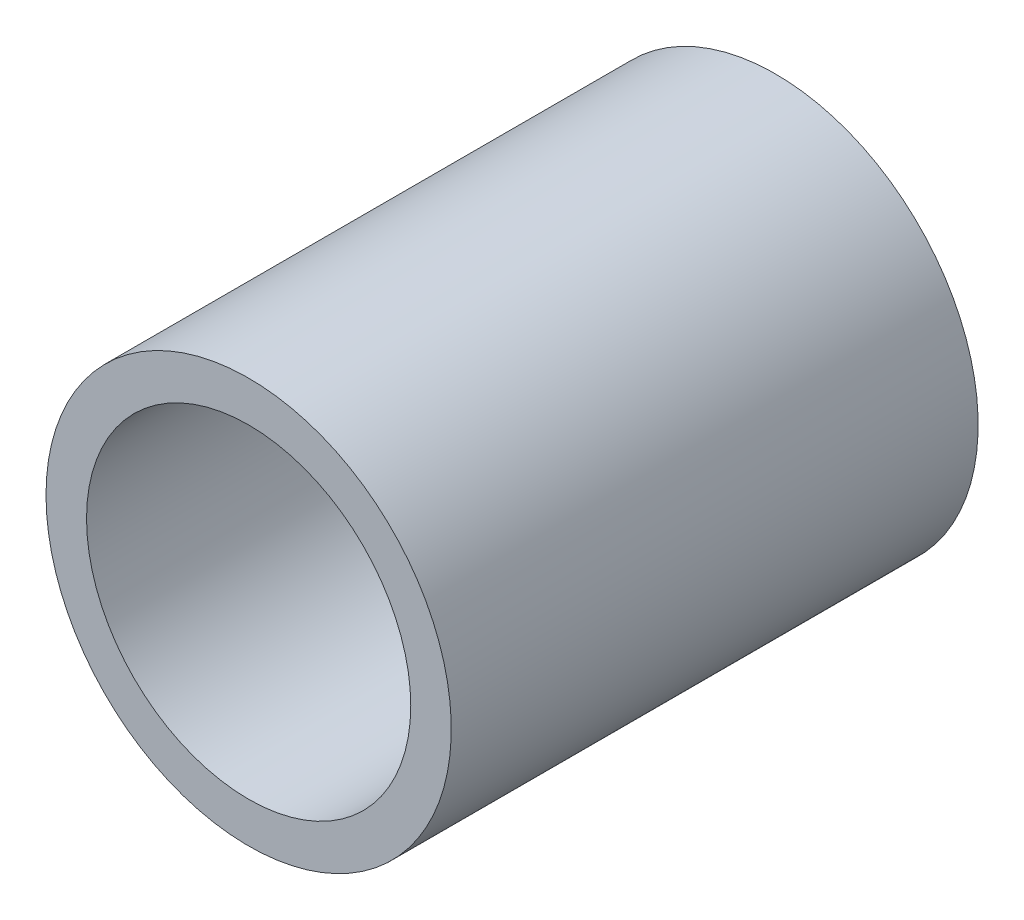
SolidWorks part; units mm, degrees
ref_plane "Front Plane" through (0, 0, 0) normal (0, 0, 1) x (1, 0, 0)
ref_plane "Top Plane" through (0, 0, 0) normal (0, 1, 0) x (1, 0, 0)
ref_plane "Right Plane" through (0, 0, 0) normal (1, 0, 0) x (0, 0, -1)
sketch "Sketch1" plane through (0, 0, 0) normal (0, 0, 1) x (1, 0, 0)
  circle A0 centre (0, 0) radius 10
  circle A1 centre (0, 0) radius 8
  dimension "D1" = 20
  dimension "D2" = 16
extrude "Boss-Extrude1" add sketch "Sketch1" along normal mid plane 26
